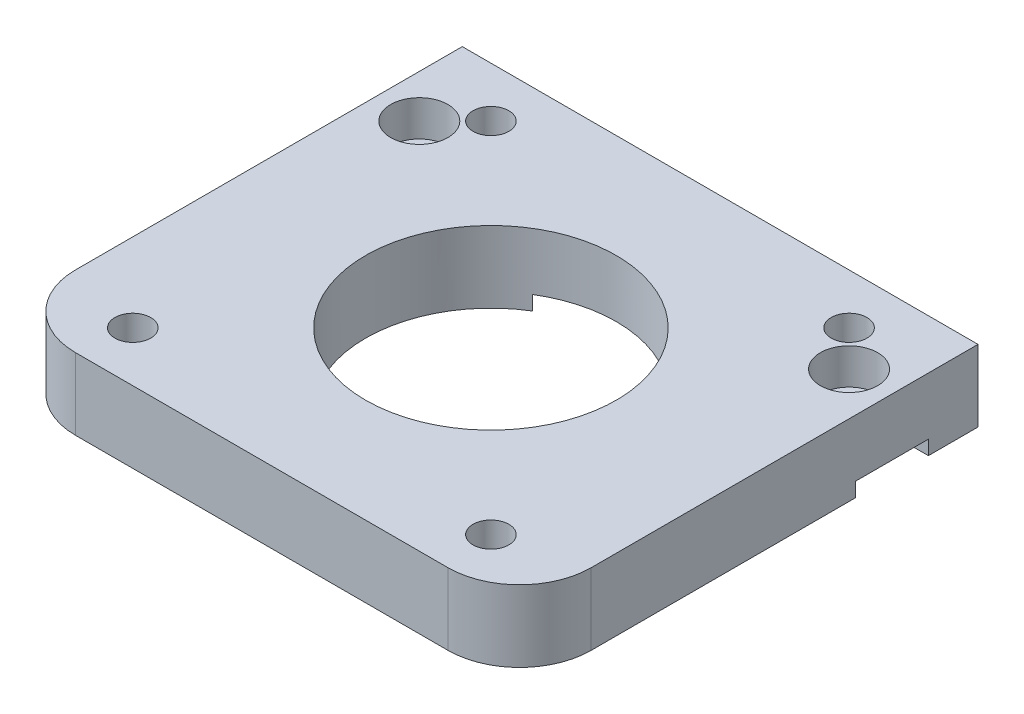
SolidWorks part; units mm, degrees
material "45钢"
ref_plane "前视基准面" through (0, 0, 0) normal (0, 0, 1) x (1, 0, 0)
ref_plane "上视基准面" through (0, 0, 0) normal (0, 1, 0) x (1, 0, 0)
ref_plane "右视基准面" through (0, 0, 0) normal (1, 0, 0) x (0, 0, -1)
sketch "草图1" plane through (0, 0, 0) normal (0, 1, 0) x (1, 0, 0)
  line L0 (0, 0) -> (103, 0)
  line L1 (103, 0) -> (103, -100)
  line L4 (103, -100) -> (0, -100)
  line L5 (0, -100) -> (0, 0)
  dimension "D1" = 103
  dimension "D2" = 100
extrude "凸台-拉伸1" add sketch "草图1" along normal blind 10
hole_wizard "Ø16.0 (16) 直径孔1" positions "草图6" profile "草图5" hole size "Ø16.0" standard "GB"
sketch "草图6" plane through (0, 15, 0) normal (0, 1, 0) x (1, 0, 0)
  line L0 (70, 0) -> (0, 0) construction
  line L2 (35, -31) -> (35, -52) construction
  line L3 (0, -52) -> (70, -52) construction
  point P0 (35, -31)
  dimension "D1" = 31
sketch "草图5" plane through (35, 15, 31) normal (1, 0, 0) x (0, 0, 1)
  line L0 (0, 0) -> (0, 15)
  line L1 (0, 15) -> (8.1, 15)
  line L2 (8.1, 15) -> (8.1, 0)
  line L5 (8.1, 0) -> (0, 0)
  line L11 (0, -6.35) -> (0, 107.95) construction
  dimension "通孔孔直径" = 16.2
  dimension "通孔孔深度" = 15
sketch "草图8" [suppressed] plane through (0, 0, 0) normal (0, -1, 0) x (1, 0, 0)
  line L1 (-59.908, 80.8452) -> (106.3415, 80.8452)
  line L2 (-59.908, 80.8452) -> (-59.908, 14)
  line L3 (-59.908, 14) -> (106.3415, 14)
  line L4 (106.3415, 80.8452) -> (106.3415, 14)
  line L5 (-59.908, 80.8452) -> (106.3415, 14) construction
  line L6 (-59.908, 14) -> (106.3415, 80.8452) construction
  circle A0 centre (35, 31) radius 8.1 construction
  point P0 (23.2167, 47.4226)
  dimension "D1" = 17
extrude "切除-拉伸3" [suppressed] cut sketch "草图8" against normal offset from surface (6 mm away) 9
ref_plane "基准面1" through (51.5, 0, 0) normal (-1, 0, 0) x (0, 0, 1)
sketch "草图9" plane through (0, 10, 0) normal (0, 1, 0) x (1, 0, 0)
  line L0 (103, 0) -> (0, 0) construction
  line L1 (0, -100) -> (15.5, -100)
  line L2 (0, -100) -> (0, -12)
  line L3 (0, -12) -> (15.5, -12)
  line L4 (15.5, -100) -> (15.5, -12)
  line L5 (103, -100) -> (87.5, -100)
  line L6 (103, -100) -> (103, -12)
  line L7 (103, -12) -> (87.5, -12)
  line L8 (87.5, -100) -> (87.5, -12)
  dimension "D1" = 72
  dimension "D2" = 12
extrude "切除-拉伸4" cut sketch "草图9" against normal through all
hole_wizard "Ø6.5 (6.5) 直径孔1" positions "草图10" profile "草图11" hole size "Ø6.5" standard "GB" end condition through all
sketch "草图10" plane through (0, 0, 12) normal (0, 0, 1) x (1, 0, 0)
  line L0 (0, 5) -> (6, 5) construction
  line L1 (0, 0) -> (0, 10) construction
  line L2 (6, 5) -> (97, 5) construction
  line L3 (97, 5) -> (103, 5) construction
  line L4 (103, 0) -> (103, 10) construction
  point P0 (6, 5)
  point P2 (97, 5)
  dimension "D1" = 6
sketch "草图11" plane through (6, 5, 12) normal (1, 0, 0) x (0, -1, 0)
  line L0 (0, 0) -> (0, 12)
  line L1 (0, 12) -> (3.25, 12)
  line L2 (3.25, 12) -> (3.25, 0)
  line L5 (3.25, 0) -> (0, 0)
  line L11 (0, -6.35) -> (0, 107.95) construction
  dimension "通孔孔直径" = 6.5
  dimension "通孔孔深度" = 12
sketch "草图12" plane through (0, 10, 0) normal (0, 1, 0) x (1, 0, 0)
  line L0 (51.5, 0) -> (51.5, -68) construction
  line L1 (103, 0) -> (0, 0) construction
  circle A0 centre (51.5, -68) radius 17.5
  dimension "D2" = 35
  dimension "D1" = 68
extrude "切除-拉伸5" cut sketch "草图12" against normal through all
fillet "圆角1" radius 10 2 edges at (15.5, 5, 100) (87.5, 5, 100)
hole_wizard "Ø5.0 (5) 直径孔1" positions "草图13" profile "草图14" hole size "Ø5.0" standard "GB"
sketch "草图13" plane through (0, 0, 0) normal (0, 0, -1) x (-1, 0, 0)
  line L0 (-51.5, 10) -> (-51.5, -2.6375) construction
  line L1 (-103, 10) -> (0, 10) construction
  line L4 (-71.5, 5) -> (-31.5, 5) construction
  line L5 (-31.5, 5) -> (0, 5) construction
  line L6 (0, 10) -> (0, 0) construction
  point P0 (-71.5, 5)
  point P2 (-31.5, 5)
  dimension "D1" = 40
sketch "草图14" plane through (71.5, 5, 0) normal (1, 0, 0) x (0, 1, 0)
  line L0 (0, 0) -> (0, 11.5022)
  line L1 (0, 11.5022) -> (2.5, 10)
  line L2 (2.5, 10) -> (2.5, 0)
  line L5 (2.5, 0) -> (0, 0)
  line L10 (0, 11.5022) -> (-2.5, 10) construction
  line L11 (0, -6.35) -> (0, 107.95) construction
  dimension "孔直径" = 5
  dimension "孔深度" = 10
  dimension "导头角度" = 118
fillet "圆角2" radius 2 2 edges at (15.5, 5, 12) (87.5, 5, 12)
sketch "草图20" plane through (0, 10, 0) normal (0, 1, 0) x (1, 0, 0)
  line L1 (112.3055, 9.6307) -> (-28.125, 9.6307)
  line L2 (112.3055, 9.6307) -> (112.3055, -36)
  line L3 (112.3055, -36) -> (-28.125, -36)
  line L4 (-28.125, 9.6307) -> (-28.125, -36)
  line L5 (25.5, -100) -> (77.5, -100) construction
  dimension "D1" = 64
extrude "切除-拉伸6" cut sketch "草图20" against normal blind 97
hole_wizard "打孔尺寸(%根据)内六角圆柱头螺钉的类型1" positions "草图23" profile "草图25" counterbore size "M4" standard "GB" end condition through all
sketch "草图23" plane through (0, 10, 0) normal (0, 1, 0) x (1, 0, 0)
  line L0 (51.5, -68) -> (51.5, -12.8239) construction
  line L2 (15.5, -36) -> (87.5, -36) construction
  point P0 (21.5, -48)
  point P2 (81.5, -48)
  dimension "D1" = 12
  dimension "D2" = 60
sketch "草图25" plane through (21.5, 10, 48) normal (1, 0, 0) x (0, 0, 1)
  line L0 (0, 0) -> (0, 10)
  line L1 (0, 10) -> (2.2, 10)
  line L3 (2.2, 10) -> (2.2, 5)
  line L4 (2.2, 5) -> (4, 5)
  line L5 (4, 5) -> (4, 0)
  line L7 (4, 0) -> (0, 0)
  line L11 (0, -6.35) -> (0, 107.95) construction
  dimension "通孔孔直径" = 4.4
  dimension "通孔孔深度" = 10
  dimension "柱形沉头孔直径" = 8
  dimension "柱形沉头孔深度" = 5
hole_wizard "M6 螺纹孔2" positions "草图26" profile "草图27" tap size "M6" standard "GB" end condition through all
sketch "草图26" plane through (0, 10, 0) normal (0, 1, 0) x (1, 0, 0)
  point P0 (26.5, -43)
  point P3 (26.5, -93)
  point P6 (76.5, -93)
  point P9 (76.5, -43)
cosmetic thread "孔螺蚊线1" parameters "D2"=6
cosmetic thread "孔螺蚊线2" parameters "D2"=6
cosmetic thread "孔螺蚊线3" parameters "D2"=6
cosmetic thread "孔螺蚊线4" parameters "D2"=6
sketch "草图27" plane through (26.5, 10, 43) normal (1, 0, 0) x (0, 0, 1)
  line L0 (0, 0) -> (0, 10)
  line L1 (0, 10) -> (2.5, 10)
  line L2 (2.5, 10) -> (2.5, 0)
  line L5 (2.5, 0) -> (0, 0)
  line L11 (0, -6.35) -> (0, 107.95) construction
  dimension "通孔螺纹孔钻头直径" = 5
  dimension "通孔螺纹孔钻头深度" = 10
sketch "草图28" plane through (0, 0, 0) normal (0, -1, 0) x (1, 0, 0)
  line L1 (-50.3404, 53.075) -> (93.3404, 53.075)
  line L2 (-50.3404, 53.075) -> (-50.3404, 42.925)
  line L3 (-50.3404, 42.925) -> (93.3404, 42.925)
  line L4 (93.3404, 53.075) -> (93.3404, 42.925)
  line L5 (-50.3404, 53.075) -> (93.3404, 42.925) construction
  line L6 (-50.3404, 42.925) -> (93.3404, 53.075) construction
  point P0 (21.5, 48)
  dimension "D1" = 10.15
extrude "切除-拉伸7" cut sketch "草图28" against normal blind 2
